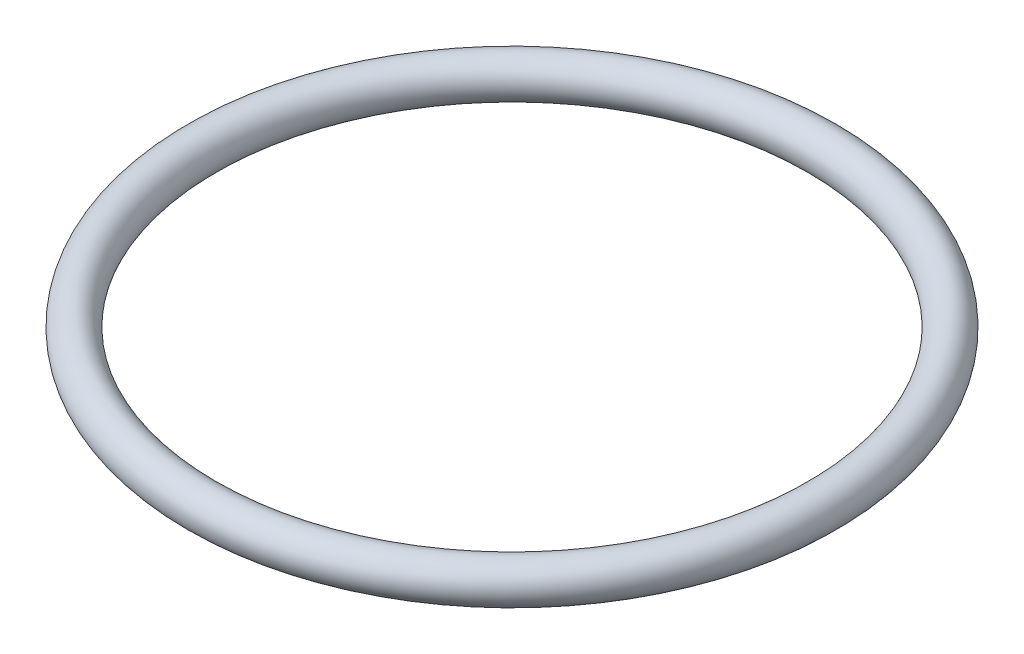
from build123d import *

# Parameters (mm, degrees)
SKETCH_1_R = 0.75


with BuildPart() as part:
    # 草图1 → 旋转1 (revolve)
    with BuildSketch(Plane.XY, mode=Mode.PRIVATE) as revolve_1_sk:
        with Locations((-11.75, 0)):
            Circle(SKETCH_1_R)
    revolve(revolve_1_sk.sketch.rotate(Axis((0, 0, 0), (0, 1, 0)), 270), axis=Axis((0, 0, 0), (0, 1, 0)))


solid = part.part
